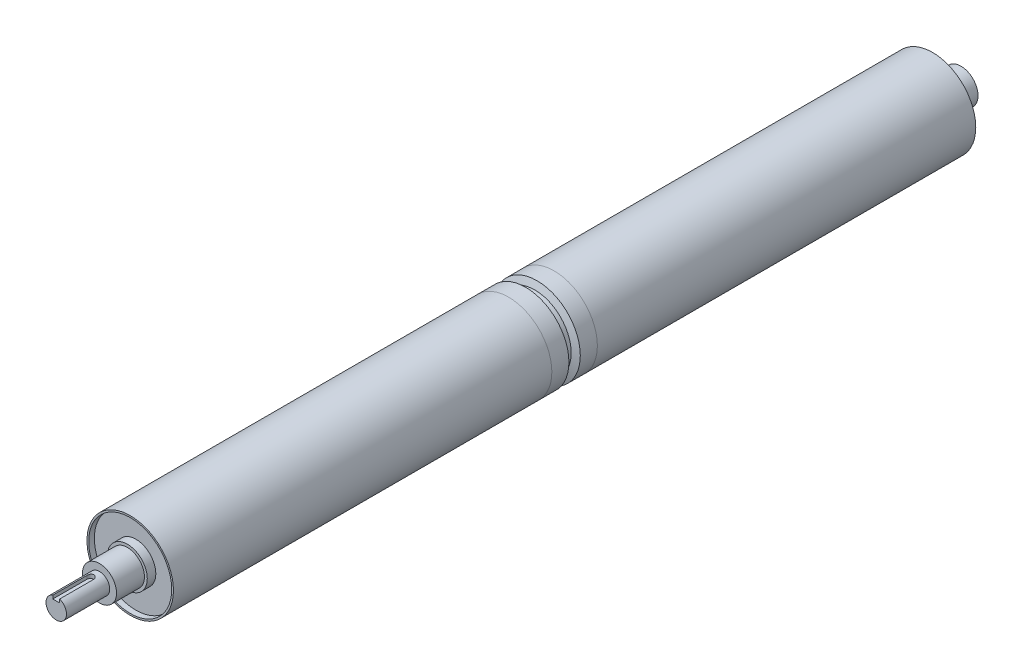
from build123d import *

# Parameters (mm, degrees)
SKETCH_1_R          = 38
SKETCH_1_R_2        = 36.5
EXTRUDE_1_DEPTH     = 352.5
EXTRUDE_START       = -5
SKETCH_2_R          = 36.5
SKETCH_2_R_2        = 17.5
EXTRUDE_2_DEPTH     = 10
SKETCH_3_R          = 36.5
SKETCH_3_R_2        = 17.5
EXTRUDE_3_DEPTH     = 10
SKETCH_10_R         = 17.5
EXTRUDE_4_DEPTH     = 377.5
SKETCH_11_R         = 17.5
EXTRUDE_5_DEPTH     = 40
SKETCH_15_R         = 23.951669513
SKETCH_15_R_2       = 15
CUT_EXTRUDE_2_DEPTH = 62.5
SKETCH_16_R         = 17.5
SKETCH_16_R_2       = 15
CUT_EXTRUDE_3_DEPTH = 22.5
SKETCH_18_R         = 54.962768961
SKETCH_18_R_2       = 24.005660026
CUT_EXTRUDE_4_DEPTH = 20
SKETCH_20_R         = 25
SKETCH_20_R_2       = 9
CUT_EXTRUDE_5_DEPTH = 38
CUT_EXTRUDE_START   = 9
CUT_EXTRUDE_1_DEPTH = 3.5


with BuildPart() as part:
    # 草图1 → 凸台-拉伸1 (new, symmetric)
    with BuildSketch(Plane.XY):
        Circle(SKETCH_1_R)
        Circle(SKETCH_1_R_2, mode=Mode.SUBTRACT)
    extrude(amount=EXTRUDE_1_DEPTH, both=True)

    # 草图18 → 切除-拉伸4 (cut, symmetric)
    with BuildSketch(Plane.XY):
        Circle(SKETCH_18_R)
        Circle(SKETCH_18_R_2, mode=Mode.SUBTRACT)
    extrude(amount=CUT_EXTRUDE_4_DEPTH, both=True, mode=Mode.SUBTRACT)


with BuildPart() as body_2:
    # 草图2 → 凸台-拉伸2 (new body)
    with BuildSketch(Plane.XY.offset(352.5).offset(EXTRUDE_START)):
        Circle(SKETCH_2_R)
        Circle(SKETCH_2_R_2, mode=Mode.SUBTRACT)
    extrude(amount=-EXTRUDE_2_DEPTH)


with BuildPart() as body_3:
    # 草图3 → 凸台-拉伸3 (new body)
    with BuildSketch(Plane(origin=(0, 0, -352.5), x_dir=(-1, 0, 0), z_dir=(0, 0, -1)).offset(EXTRUDE_START)):
        Circle(SKETCH_3_R)
        Circle(SKETCH_3_R_2, mode=Mode.SUBTRACT)
    extrude(amount=-EXTRUDE_3_DEPTH)


with BuildPart() as body_4:
    # 草图10 → 凸台-拉伸4 (new, symmetric)
    with BuildSketch(Plane.XY):
        Circle(SKETCH_10_R)
    extrude(amount=EXTRUDE_4_DEPTH, both=True)

    # 草图11 → 凸台-拉伸5 (add)
    with BuildSketch(Plane.XY.offset(377.5)):
        Circle(SKETCH_11_R)
    extrude(amount=EXTRUDE_5_DEPTH)

    # 草图15 → 切除-拉伸2 (cut)
    with BuildSketch(Plane.XY.offset(417.5)):
        Circle(SKETCH_15_R)
        Circle(SKETCH_15_R_2, mode=Mode.SUBTRACT)
    extrude(amount=-CUT_EXTRUDE_2_DEPTH, mode=Mode.SUBTRACT)

    # 草图16 → 切除-拉伸3 (cut)
    with BuildSketch(Plane(origin=(0, 0, -377.5), x_dir=(-1, 0, 0), z_dir=(0, 0, -1))):
        Circle(SKETCH_16_R)
        with Locations(Location((0, 0, 0), (0, 0, 180))):
            Circle(SKETCH_16_R_2, mode=Mode.SUBTRACT)
    extrude(amount=-CUT_EXTRUDE_3_DEPTH, mode=Mode.SUBTRACT)

    # 草图20 → 切除-拉伸5 (cut)
    with BuildSketch(Plane.XY.offset(417.5)):
        Circle(SKETCH_20_R)
        Circle(SKETCH_20_R_2, mode=Mode.SUBTRACT)
    extrude(amount=-CUT_EXTRUDE_5_DEPTH, mode=Mode.SUBTRACT)

    # 草图14 → 切除-拉伸1 (cut)
    with BuildSketch(Plane(origin=(0, 0, 0), x_dir=(1, 0, 0), z_dir=(0, 1, 0)).offset(CUT_EXTRUDE_START)):
        with BuildLine():
            Line((-3, -417.5), (-3, -387.5))
            ThreePointArc((-3, -387.5), (0, -384.5), (3, -387.5))
            Line((3, -387.5), (3, -417.5))
            ThreePointArc((3, -417.5), (0, -420.5), (-3, -417.5))
        make_face()
    extrude(amount=-CUT_EXTRUDE_1_DEPTH, mode=Mode.SUBTRACT)


with BuildPart() as cut_extrude_4_piece_1:
    # of the separate pieces the step leaves, piece 1, a body of its own (cut_extrude_4_pieces)
    add(part.part.solids().sort_by_distance((38, 0, -352.5))[0])


with BuildPart() as cut_extrude_4_piece_2:
    # of the separate pieces the step leaves, piece 2, a body of its own (cut_extrude_4_pieces)
    add(part.part.solids().sort_by_distance((38, 0, 20))[0])


with BuildPart() as body_6:
    # 草图19 → 旋转2 (revolve)
    with BuildSketch(Plane(origin=(0, 0, 0), x_dir=(1, 0, 0), z_dir=(0, 1, 0)), mode=Mode.PRIVATE) as revolve_2_sk:
        Polygon((-36.5, 30), (-36.5, 20), (-38, 20), (-38, -20), (-36.5, -20), (-36.5, -30), (-17.5, -30), (-17.5, 30), align=None)
    revolve(revolve_2_sk.sketch.rotate(Axis((0, 0, 0), (0, 0, -1)), 180), axis=Axis((0, 0, 0), (0, 0, -1)))

    # 草图17 → 切除-旋转5 (revolve, cut)
    with BuildSketch(Plane(origin=(0, 0, 0), x_dir=(1, 0, 0), z_dir=(0, 1, 0)), mode=Mode.PRIVATE) as cut_revolve_5_sk:
        Polygon((32, 3), (32, -3), (38, -5), (38, 5), align=None)
    revolve(cut_revolve_5_sk.sketch.rotate(Axis((0, 0, 0), (0, 0, 1)), 180), axis=Axis((0, 0, 0), (0, 0, 1)), mode=Mode.SUBTRACT)


solid = Compound([body_2.part, body_3.part, body_4.part, cut_extrude_4_piece_1.part, cut_extrude_4_piece_2.part, body_6.part])
